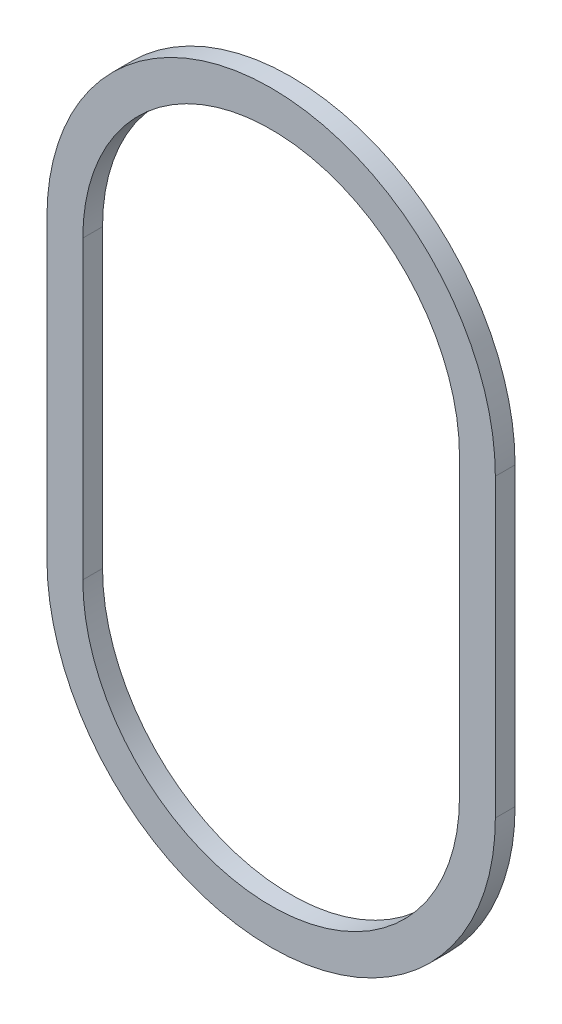
from build123d import *

# Parameters (mm, degrees)
BOSS_EXTRUDE1_DEPTH = 2.2


with BuildPart() as part:
    # Sketch1 → Boss-Extrude1 (new body)
    with BuildSketch(Plane.XY):
        with BuildLine():
            Line((-25, 0), (-25, 33))
            ThreePointArc((-25, 33), (0, 58), (25, 33))
            Line((25, 33), (25, 0))
            ThreePointArc((25, 0), (0, -25), (-25, 0))
        make_face()
        with BuildLine():
            Line((-21, 0), (-21, 33))
            ThreePointArc((-21, 33), (0, 54), (21, 33))
            Line((21, 33), (21, 0))
            ThreePointArc((21, 0), (0, -21), (-21, 0))
        make_face(mode=Mode.SUBTRACT)
    extrude(amount=BOSS_EXTRUDE1_DEPTH)


solid = part.part
